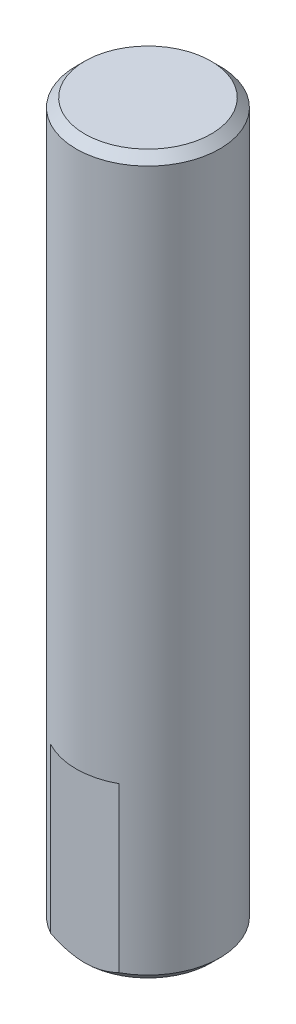
SolidWorks part; units mm, degrees
ref_plane "Front Plane" through (0, 0, 0) normal (0, 0, 1) x (1, 0, 0)
ref_plane "Top Plane" through (0, 0, 0) normal (0, 1, 0) x (1, 0, 0)
ref_plane "Right Plane" through (0, 0, 0) normal (1, 0, 0) x (0, 0, -1)
sketch "Sketch1" plane through (0, 0, 0) normal (0, 1, 0) x (1, 0, 0)
  circle A0 centre (0, 0) radius 2.5
  dimension "D1" = 5
extrude "Boss-Extrude1" add sketch "Sketch1" along normal blind 25
chamfer "Chamfer1" distance 0.3 angle 45 2 edges at (0, 0, 2.5) (0, 25, 2.5)
sketch "Sketch3" plane through (0, 0, 0) normal (0, -1, 0) x (1, 0, 0)
  line L0 (0, 0) -> (0, -50000) construction
  line L2 (-2.0161, 2.8) -> (2.0161, 2.8)
  line L3 (-2.0161, 2.8) -> (-2.0161, 2.2)
  line L4 (-2.0161, 2.2) -> (2.0161, 2.2)
  line L5 (2.0161, 2.8) -> (2.0161, 2.2)
  line L6 (-2.0161, 2.8) -> (2.0161, 2.2) construction
  line L7 (-2.0161, 2.2) -> (2.0161, 2.8) construction
  circle A0 centre (0, 0) radius 2.5 construction
  point P3 (0, 2.5)
  dimension "D1" = 2.2
extrude "Cut-Extrude2" cut sketch "Sketch3" against normal blind 6
